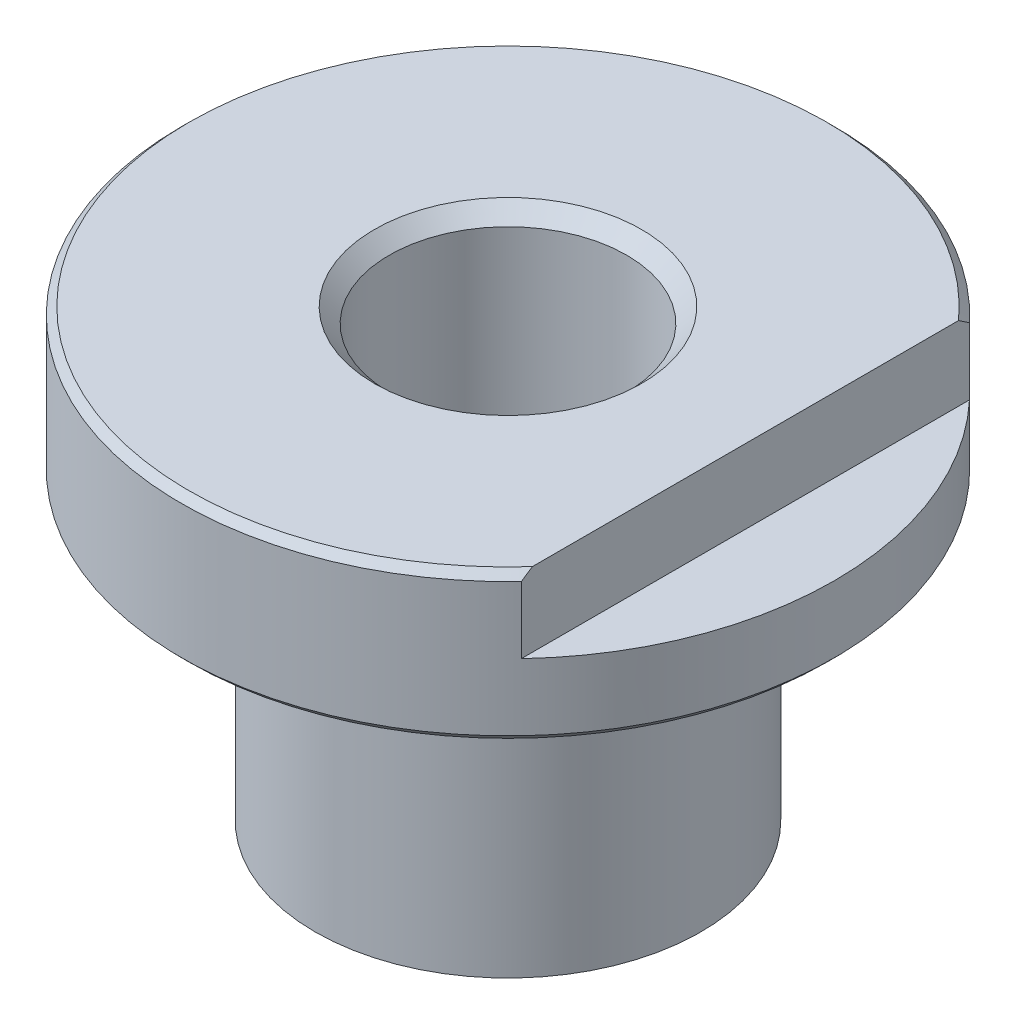
SolidWorks part; units mm, degrees
ref_plane "Front Plane" through (0, 0, 0) normal (0, 0, 1) x (1, 0, 0)
ref_plane "Top Plane" through (0, 0, 0) normal (0, 1, 0) x (1, 0, 0)
ref_plane "Right Plane" through (0, 0, 0) normal (1, 0, 0) x (0, 0, -1)
sketch "Sketch1" plane through (0, 0, 0) normal (0, 0, 1) x (1, 0, 0)
  line L0 (0, 40.8114) -> (0, -20.5963) construction
  line L1 (-22, 18.5319) -> (-22, 8.5319)
  line L2 (-22, 8.5319) -> (-13, 8.5319)
  line L3 (-13, 8.5319) -> (-13, -11.4681)
  line L4 (-13, -11.4681) -> (-8, -11.4681)
  line L5 (-8, -11.4681) -> (-8, 18.5319)
  line L6 (-8, 18.5319) -> (-22, 18.5319)
  dimension "D1" = 8
  dimension "D2" = 13
  dimension "D3" = 20
  dimension "D4" = 10
  dimension "D5" = 22
revolve "Revolve1" add sketch "Sketch1" angle 360 about L0
chamfer "Chamfer1" distance 0.5 angle 45 2 edges at (0, 8.5319, 22) (0, 18.5319, 22)
chamfer "Chamfer2" distance 1 angle 45 1 edges at (0, 18.5319, 8)
sketch "Sketch2" plane through (0, 18.5319, 0) normal (0, 1, 0) x (1, 0, 0)
  line L1 (16, 25.0172) -> (36.2237, 25.0172)
  line L2 (16, 25.0172) -> (16, -26.8367)
  line L3 (16, -26.8367) -> (36.2237, -26.8367)
  line L4 (36.2237, 25.0172) -> (36.2237, -26.8367)
  dimension "D1" = 16
extrude "Cut-Extrude1" cut sketch "Sketch2" against normal blind 5
